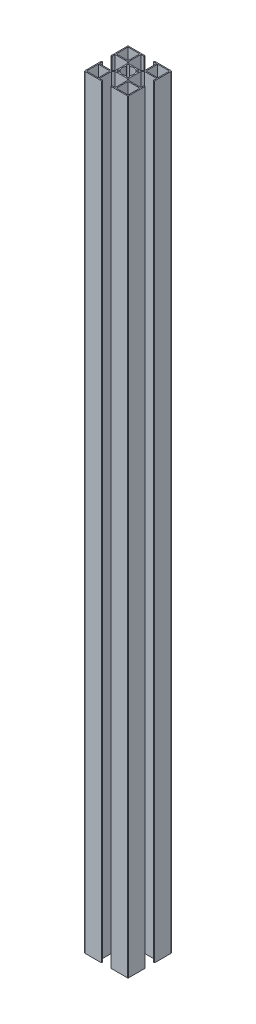
SolidWorks part; units mm, degrees
material "6061 Aluminium alloy"
ref_plane "Front" through (0, 0, 0) normal (0, 0, 1) x (1, 0, 0)
ref_plane "Top" through (0, 0, 0) normal (0, 1, 0) x (1, 0, 0)
ref_plane "Right" through (0, 0, 0) normal (1, 0, 0) x (0, 0, -1)
sketch "Sketch1" plane through (0, 0, 0) normal (0, 1, 0) x (1, 0, 0)
  line L0 (0, 0) -> (0, 20) construction
  line L1 (0, 0) -> (-20, 0) construction
  line L2 (-4.3, 20) -> (-19.5, 20)
  line L3 (-20, 19.5) -> (-20, 4.3)
  line L4 (-20, 4.3) -> (-19.05, 4.3)
  line L5 (-19.05, 4.3) -> (-19.05, 7.25)
  line L6 (-19.05, 7.25) -> (-7.9218, 7.25)
  line L7 (0, 0) -> (-4.3841, 4.3841) construction
  line L8 (-4.3, 20) -> (-4.3, 19.05)
  line L9 (-4.3, 19.05) -> (-7.25, 19.05)
  line L10 (-7.25, 19.05) -> (-7.25, 7.9218)
  line L11 (-7.25, 7.9218) -> (-5.5282, 6.2)
  line L12 (-8.2, 19.05) -> (-19.05, 19.05)
  line L13 (-19.05, 19.05) -> (-19.05, 8.2)
  line L14 (-19.05, 8.2) -> (-8.2, 8.2)
  line L15 (-7.9218, 7.25) -> (-6.2, 5.5282)
  line L16 (-8.2, 19.05) -> (-8.2, 8.2)
  line L17 (-5.5282, 6.2) -> (0, 6.2)
  line L18 (-6.2, 5.5282) -> (-6.2, 0)
  line L19 (-5.0912, 3.677) -> (-4.3875, 2.9732)
  line L20 (-3.677, 5.0912) -> (-2.9732, 4.3875)
  line L21 (0, 6.2) -> (0, 5.3)
  line L22 (-5.3, 0) -> (-6.2, 0)
  arc A0 (-4.3875, 2.9732) -> (-5.3, 0) centre (0, 0) ccw
  arc A1 (-19.5, 20) -> (-20, 19.5) centre (-19.5, 19.5) ccw
  circle A2 centre (0, 0) radius 7.2 construction
  arc A3 (-3.677, 5.0912) -> (-5.0912, 3.677) centre (-4.3841, 4.3841) ccw
  arc A4 (0, 5.3) -> (-2.9732, 4.3875) centre (0, 0) ccw
  dimension "D1" = 10.6
  dimension "D5" = 0.5
  dimension "D17" = 14.4
  dimension "D18" = 2
  dimension "D2" = 40
  dimension "D3" = 40
  dimension "D4" = 8.6
  dimension "D6" = 0.95
  dimension "D7" = 8.6
  dimension "D8" = 14.5
  dimension "D9" = 0.95
  dimension "D10" = 0.95
  dimension "D11" = 0.95
  dimension "D12" = 0.95
  dimension "D13" = 14.5
  dimension "D14" = 13.8
  dimension "D15" = 45
  dimension "D16" = 13.8
extrude "Boss-Extrude1" add sketch "Sketch1" along normal blind 700
mirror "Mirror1" about plane through (0, 0, 0) normal (1, 0, 0) of "Boss-Extrude1"
mirror "Mirror2" about plane through (0, 0, 0) normal (0, 0, 1) of "Mirror1", "Boss-Extrude1"
ref_plane "Plane1" through (0, 350, 0) normal (0, 1, 0) x (1, 0, 0)
